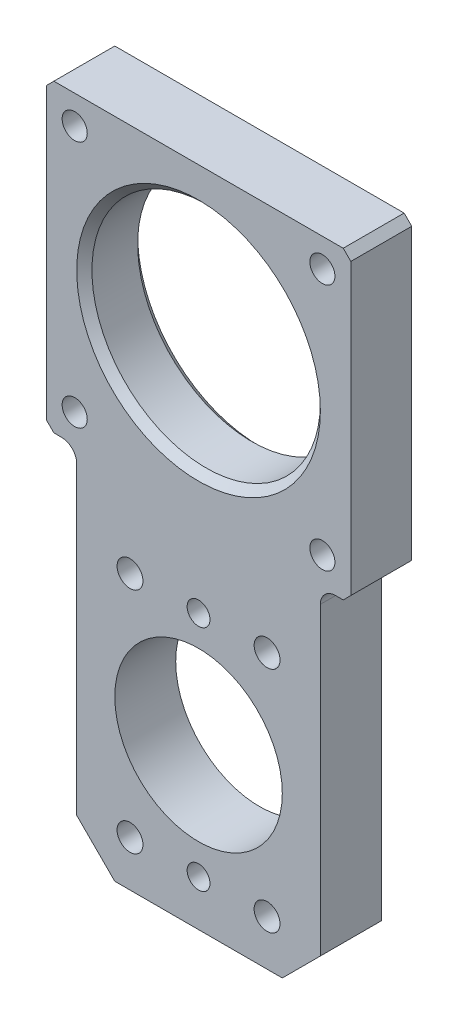
SolidWorks part; units mm, degrees
material "A6063"
ref_plane "Front Plane" through (0, 0, 0) normal (0, 0, 1) x (1, 0, 0)
ref_plane "Top Plane" through (0, 0, 0) normal (0, 1, 0) x (1, 0, 0)
ref_plane "Right Plane" through (0, 0, 0) normal (1, 0, 0) x (0, 0, -1)
sketch "Sketch1" plane through (0, 0, 0) normal (0, 0, 1) x (1, 0, 0)
  line L0 (0, 0) -> (0, -42.4581) construction
  line L1 (-20, -43.5) -> (20, -43.5)
  line L2 (-20, -43.5) -> (-20, 43.5)
  line L3 (-20, 43.5) -> (20, 43.5)
  line L4 (20, -43.5) -> (20, 43.5)
  line L5 (-20, -43.5) -> (20, 43.5) construction
  line L6 (-20, 43.5) -> (20, -43.5) construction
  line L7 (20, -43.5) -> (16, -43.5)
  line L8 (20, -43.5) -> (20, 3.5)
  line L9 (20, 3.5) -> (16, 3.5)
  line L10 (16, -43.5) -> (16, 3.5)
  line L11 (-20, -43.5) -> (-16, -43.5)
  line L12 (-20, -43.5) -> (-20, 3.5)
  line L13 (-20, 3.5) -> (-16, 3.5)
  line L14 (-16, -43.5) -> (-16, 3.5)
  point P0 (0, 0)
  dimension "D1" = 87
  dimension "D2" = 40
  dimension "D3" = 40
  dimension "D4" = 32
extrude "Boss-Extrude1" add sketch "Sketch1" along normal mid plane 8 contours L14 L1 L10 L9 L4 L3 L2 L13
hole_wizard "M4 Tapped Hole1" positions "Sketch3" profile "Sketch2" tap size "M4" standard "GB" end condition up to next
sketch "Sketch3" plane through (0, 0, 4) normal (0, 0, 1) x (1, 0, 0)
  line L1 (-20, 23.5) -> (20, 23.5) construction
  line L2 (-20, 3.5) -> (-20, 43.5) construction
  line L3 (20, 3.5) -> (20, 43.5) construction
  line L6 (-16.2635, 7.2365) -> (16.2635, 39.7635) construction
  circle A0 centre (0, 23.5) radius 23 construction
  point P0 (-16.2635, 39.7635)
  point P2 (16.2635, 39.7635)
  point P4 (16.2635, 7.2365)
  point P6 (-16.2635, 7.2365)
  dimension "D1" = 46
  dimension "D2" = 45
sketch "Sketch2" plane through (-16.2635, 39.7635, 4) normal (1, 0, 0) x (0, -1, 0)
  line L0 (0, 0) -> (0, 8)
  line L1 (0, 8) -> (1.65, 8)
  line L2 (1.65, 8) -> (1.65, 0)
  line L5 (1.65, 0) -> (0, 0)
  line L11 (0, -6.35) -> (0, 107.95) construction
  dimension "通孔螺纹孔钻头直径" = 3.3
  dimension "通孔螺纹孔钻头深度" = 8
cosmetic thread "Cosmetic Thread 1" parameters "D2"=4
cosmetic thread "Cosmetic Thread 2" parameters "D2"=4
cosmetic thread "Cosmetic Thread 3" parameters "D2"=4
cosmetic thread "Cosmetic Thread 4" parameters "D2"=4
hole_wizard "M3 Clearance Hole1" positions "Sketch5" profile "Sketch4" hole size "M3" standard "GB" end condition up to next
sketch "Sketch5" plane through (0, 0, 4) normal (0, 0, 1) x (1, 0, 0)
  line L0 (20, 3.5) -> (16, 3.5) construction
  line L1 (0, 0) -> (0, -41.5287) construction
  point P0 (-9, -7.5)
  point P2 (9, -7.5)
  point P4 (9, -37.5)
  point P6 (-9, -37.5)
  dimension "D1" = 11
  dimension "D2" = 18
  dimension "D3" = 30
sketch "Sketch4" plane through (-9, -7.5, 4) normal (1, 0, 0) x (0, -1, 0)
  line L0 (0, 0) -> (0, 8)
  line L1 (0, 8) -> (1.7, 8)
  line L2 (1.7, 8) -> (1.7, 0)
  line L5 (1.7, 0) -> (0, 0)
  line L11 (0, -6.35) -> (0, 107.95) construction
  dimension "通孔孔直径" = 3.4
  dimension "通孔孔深度" = 8
sketch "Sketch6" plane through (0, 0, 4) normal (0, 0, 1) x (1, 0, 0)
  line L0 (-9, -7.5) -> (9, -7.5) construction
  line L1 (-16.2635, 7.2365) -> (16.2635, 7.2365) construction
  line L2 (-16.2635, 7.2365) -> (-16.2635, 39.7635) construction
  line L3 (-16.2635, 39.7635) -> (16.2635, 39.7635) construction
  line L4 (16.2635, 7.2365) -> (16.2635, 39.7635) construction
  line L5 (-16.2635, 7.2365) -> (16.2635, 39.7635) construction
  line L6 (-16.2635, 39.7635) -> (16.2635, 7.2365) construction
  line L7 (-9, -37.5) -> (9, -37.5) construction
  line L8 (0, -7.5) -> (0, -37.5) construction
  circle A0 centre (0, 23.5) radius 15
  circle A1 centre (0, -7.5) radius 1.5
  circle A2 centre (0, -37.5) radius 1.5
  circle A3 centre (0, -22.5) radius 11
  point P0 (0, 23.5)
  dimension "D1" = 30
  dimension "D2" = 3
  dimension "D3" = 22
extrude "Cut-Extrude1" cut sketch "Sketch6" against normal through all
chamfer "Chamfer1" distance 5 angle 45 2 edges at (-16, -43.5, 0) (16, -43.5, 0)
chamfer "Chamfer2" distance 1 angle 45 6 edges at (15, 23.5, -4) (15, 23.5, 4) (-20, 43.5, 0) (20, 43.5, 0) (-20, 3.5, 0) (20, 3.5, 0)
fillet "Fillet1" radius 2 2 edges at (-16, 3.5, 0) (16, 3.5, 0)
